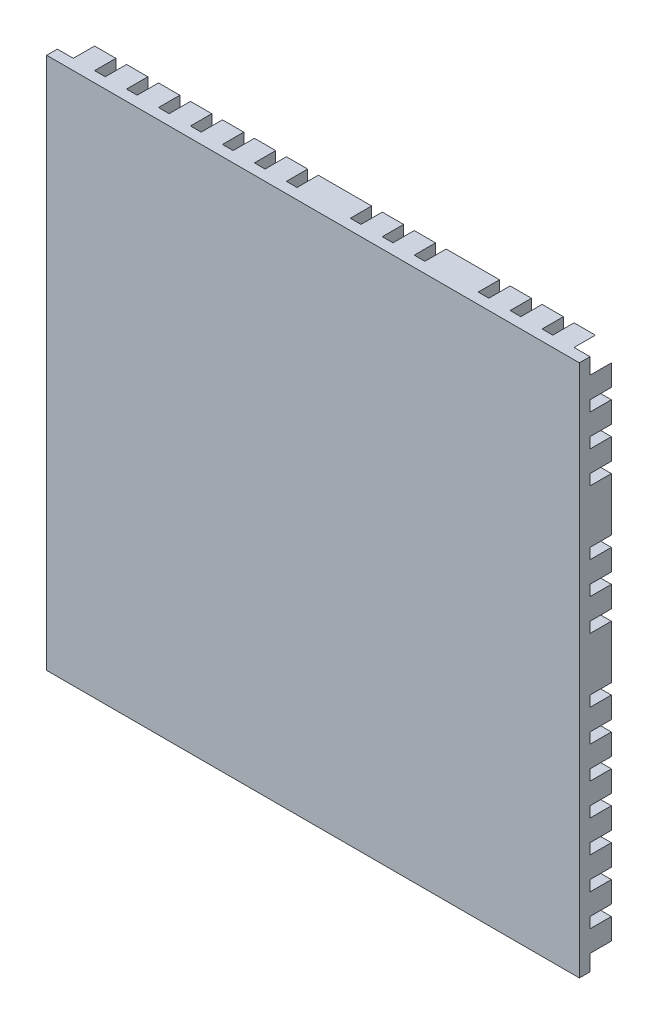
from build123d import *

# Parameters (mm, degrees)
BOSS_EXTRUDE3_DEPTH = 1
SKETCH2_W           = 50
SKETCH2_H           = 50
BOSS_EXTRUDE4_DEPTH = 3
CUT_EXTRUDE1_DEPTH  = 3


with BuildPart() as part:
    # Sketch1 → Boss-Extrude3 (new body)
    with BuildSketch(Plane.XY):
        Polygon((-25, -25), (-23.5, -25), (-21.5, -23), (-21.5, -25), (-20.5, -25), (-20.5, -22), (-18.5, -20), (-18.5, -25), (-17.5, -25), (-17.5, -19), (-15.5, -17), (-15.5, -25), (-14.5, -25), (-14.5, -16), (-12.5, -14), (-12.5, -25.000006046), (-11.5, -25.000006046), (-11.5, -13), (-9.5, -11), (-9.5, -25.000006046), (-8.5, -25.000006046), (-8.5, -10), (-6.5, -8), (-6.5, -25.000006046), (-5.5, -25.000006046), (-5.5, -7), (-3.5, -5), (-3.5, -25.000006046), (-2.5, -25.000006046), (-2.5, -4), (0, -1.5), (2.5, -4), (2.5, -25.000006046), (3.5, -25.000006046), (3.5, -5), (5.5, -7), (5.5, -25.000006046), (6.5, -25.000006046), (6.5, -8), (8.5, -10), (8.5, -25.000006046), (9.5, -25.000006046), (9.5, -11), (11.5, -13), (11.5, -25.000006046), (12.5, -25.000006046), (12.5, -14), (14.5, -16), (14.5, -25), (15.5, -25), (15.5, -17), (17.5, -19), (17.5, -25), (18.5, -25), (18.5, -20), (20.5, -22), (20.5, -25), (21.5, -25), (21.5, -23), (23.5, -25), (25, -25), (25, -23.5), (23, -21.5), (25, -21.5), (25, -20.5), (22, -20.5), (20, -18.5), (25, -18.5), (25, -17.5), (19, -17.5), (17, -15.5), (25, -15.5), (25, -14.5), (16, -14.5), (14, -12.5), (25.000006046, -12.5), (25.000006046, -11.5), (13, -11.5), (11, -9.5), (25.000006046, -9.5), (25.000006046, -8.5), (10, -8.5), (8, -6.5), (25.000006046, -6.5), (25.000006046, -5.5), (7, -5.5), (5, -3.5), (25.000006046, -3.5), (25.000006046, -2.5), (4, -2.5), (1.5, 0), (4, 2.5), (25.000006046, 2.5), (25.000006046, 3.5), (5, 3.5), (7, 5.5), (25.000006046, 5.5), (25.000006046, 6.5), (8, 6.5), (10, 8.5), (25.000006046, 8.5), (25.000006046, 9.5), (11, 9.5), (16, 14.5), (25, 14.5), (25, 15.5), (17, 15.5), (19, 17.5), (25, 17.5), (25, 18.5), (20, 18.5), (22, 20.5), (25, 20.5), (25, 21.5), (23, 21.5), (25, 23.5), (25, 25), (23.5, 25), (21.5, 23), (21.5, 25), (20.5, 25), (20.5, 22), (18.5, 20), (18.5, 25), (17.5, 25), (17.5, 19), (15.5, 17), (15.5, 25), (14.5, 25), (14.5, 16), (9.5, 11), (9.5, 25.000006046), (8.5, 25.000006046), (8.5, 10), (6.5, 8), (6.5, 25.000006046), (5.5, 25.000006046), (5.5, 7), (3.5, 5), (3.5, 25.000006046), (2.5, 25.000006046), (2.5, 4), (0, 1.5), (-2.5, 4), (-2.5, 25.000006046), (-3.5, 25.000006046), (-3.5, 5), (-5.5, 7), (-5.5, 25.000006046), (-6.5, 25.000006046), (-6.5, 8), (-8.5, 10), (-8.5, 25.000006046), (-9.5, 25.000006046), (-9.5, 11), (-11.5, 13), (-11.5, 25.000006046), (-12.5, 25.000006046), (-12.5, 14), (-14.5, 16), (-14.5, 25), (-15.5, 25), (-15.5, 17), (-17.5, 19), (-17.5, 25), (-18.5, 25), (-18.5, 20), (-20.5, 22), (-20.5, 25), (-21.5, 25), (-21.5, 23), (-23.5, 25), (-25, 25), (-25, 23.5), (-23, 21.5), (-25, 21.5), (-25, 20.5), (-22, 20.5), (-20, 18.5), (-25, 18.5), (-25, 17.5), (-19, 17.5), (-17, 15.5), (-25, 15.5), (-25, 14.5), (-16, 14.5), (-14, 12.5), (-25.000006046, 12.5), (-25.000006046, 11.5), (-13, 11.5), (-11, 9.5), (-25.000006046, 9.5), (-25.000006046, 8.5), (-10, 8.5), (-8, 6.5), (-25.000006046, 6.5), (-25.000006046, 5.5), (-7, 5.5), (-5, 3.5), (-25.000006046, 3.5), (-25.000006046, 2.5), (-4, 2.5), (-1.5, 0), (-4, -2.5), (-25.000006046, -2.5), (-25.000006046, -3.5), (-5, -3.5), (-7, -5.5), (-25.000006046, -5.5), (-25.000006046, -6.5), (-8, -6.5), (-10, -8.5), (-25.000006046, -8.5), (-25.000006046, -9.5), (-11, -9.5), (-13, -11.5), (-25.000006046, -11.5), (-25.000006046, -12.5), (-14, -12.5), (-16, -14.5), (-25, -14.5), (-25, -15.5), (-17, -15.5), (-19, -17.5), (-25, -17.5), (-25, -18.5), (-20, -18.5), (-22, -20.5), (-25, -20.5), (-25, -21.5), (-23, -21.5), (-25, -23.5), align=None)
    extrude(amount=BOSS_EXTRUDE3_DEPTH)


with BuildPart() as body_2:
    # Sketch2 → Boss-Extrude4 (new body)
    with BuildSketch(Plane.XY.offset(1)):
        Rectangle(SKETCH2_W, SKETCH2_H)
    extrude(amount=BOSS_EXTRUDE4_DEPTH)


with BuildPart() as cut_extrude1_tool:
    # Sketch3 → Cut-Extrude1 (new body)
    with BuildSketch(Plane(origin=(0, 0, 0), x_dir=(-1, 0, 0), z_dir=(0, 0, -1))):
        Polygon((20.5, -22), (20.5, -25), (21.5, -25), (21.5, -23), (23.5, -25), (25, -25), (25, -23.5), (23, -21.5), (25, -21.5), (25, -20.5), (22, -20.5), (20, -18.5), (25, -18.5), (25, -17.5), (19, -17.5), (17, -15.5), (25, -15.5), (25, -14.5), (16, -14.5), (14, -12.5), (25.000006046, -12.5), (25.000006046, -11.5), (13, -11.5), (11, -9.5), (25.000006046, -9.5), (25.000006046, -8.5), (10, -8.5), (8, -6.5), (25.000006046, -6.5), (25.000006046, -5.5), (7, -5.5), (5, -3.5), (25.000006046, -3.5), (25.000006046, -2.5), (4, -2.5), (1.5, 0), (4, 2.5), (25.000006046, 2.5), (25.000006046, 3.5), (5, 3.5), (7, 5.5), (25.000006046, 5.5), (25.000006046, 6.5), (8, 6.5), (10, 8.5), (25.000006046, 8.5), (25.000006046, 9.5), (11, 9.5), (13, 11.5), (25.000006046, 11.5), (25.000006046, 12.5), (14, 12.5), (16, 14.5), (25, 14.5), (25, 15.5), (17, 15.5), (19, 17.5), (25, 17.5), (25, 18.5), (20, 18.5), (22, 20.5), (25, 20.5), (25, 21.5), (23, 21.5), (25, 23.5), (25, 25), (23.5, 25), (21.5, 23), (21.5, 25), (20.5, 25), (20.5, 22), (18.5, 20), (18.5, 25), (17.5, 25), (17.5, 19), (15.5, 17), (15.5, 25), (14.5, 25), (14.5, 16), (12.5, 14), (12.5, 25.000006046), (11.5, 25.000006046), (11.5, 13), (9.5, 11), (9.5, 25.000006046), (8.5, 25.000006046), (8.5, 10), (6.5, 8), (6.5, 25.000006046), (5.5, 25.000006046), (5.5, 7), (3.5, 5), (3.5, 25.000006046), (2.5, 25.000006046), (2.5, 4), (0, 1.5), (-2.5, 4), (-2.5, 25.000006046), (-3.5, 25.000006046), (-3.5, 5), (-5.5, 7), (-5.5, 25.000006046), (-6.5, 25.000006046), (-6.5, 8), (-8.5, 10), (-8.5, 25.000006046), (-9.5, 25.000006046), (-9.5, 11), (-14.5, 16), (-14.5, 25), (-15.5, 25), (-15.5, 17), (-17.5, 19), (-17.5, 25), (-18.5, 25), (-18.5, 20), (-20.5, 22), (-20.5, 25), (-21.5, 25), (-21.5, 23), (-23.5, 25), (-25, 25), (-25, 23.5), (-23, 21.5), (-25, 21.5), (-25, 20.5), (-22, 20.5), (-20, 18.5), (-25, 18.5), (-25, 17.5), (-19, 17.5), (-17, 15.5), (-25, 15.5), (-25, 14.5), (-16, 14.5), (-11, 9.5), (-25.000006046, 9.5), (-25.000006046, 8.5), (-10, 8.5), (-8, 6.5), (-25.000006046, 6.5), (-25.000006046, 5.5), (-7, 5.5), (-5, 3.5), (-25.000006046, 3.5), (-25.000006046, 2.5), (-4, 2.5), (-1.5, 0), (-4, -2.5), (-25.000006046, -2.5), (-25.000006046, -3.5), (-5, -3.5), (-7, -5.5), (-25.000006046, -5.5), (-25.000006046, -6.5), (-8, -6.5), (-10, -8.5), (-25.000006046, -8.5), (-25.000006046, -9.5), (-11, -9.5), (-13, -11.5), (-25.000006046, -11.5), (-25.000006046, -12.5), (-14, -12.5), (-16, -14.5), (-25, -14.5), (-25, -15.5), (-17, -15.5), (-19, -17.5), (-25, -17.5), (-25, -18.5), (-20, -18.5), (-22, -20.5), (-25, -20.5), (-25, -21.5), (-23, -21.5), (-25, -23.5), (-25, -25), (-23.5, -25), (-21.5, -23), (-21.5, -25), (-20.5, -25), (-20.5, -22), (-18.5, -20), (-18.5, -25), (-17.5, -25), (-17.5, -19), (-15.5, -17), (-15.5, -25), (-14.5, -25), (-14.5, -16), (-12.5, -14), (-12.5, -25.000006046), (-11.5, -25.000006046), (-11.5, -13), (-9.5, -11), (-9.5, -25.000006046), (-8.5, -25.000006046), (-8.5, -10), (-6.5, -8), (-6.5, -25.000006046), (-5.5, -25.000006046), (-5.5, -7), (-3.5, -5), (-3.5, -25.000006046), (-2.5, -25.000006046), (-2.5, -4), (0, -1.5), (2.5, -4), (2.5, -25.000006046), (3.5, -25.000006046), (3.5, -5), (5.5, -7), (5.5, -25.000006046), (6.5, -25.000006046), (6.5, -8), (8.5, -10), (8.5, -25.000006046), (9.5, -25.000006046), (9.5, -11), (11.5, -13), (11.5, -25.000006046), (12.5, -25.000006046), (12.5, -14), (14.5, -16), (14.5, -25), (15.5, -25), (15.5, -17), (17.5, -19), (17.5, -25), (18.5, -25), (18.5, -20), align=None)
    extrude(amount=-CUT_EXTRUDE1_DEPTH)


with BuildPart() as part_1:
    add(part.part)

    # Cut-Extrude1: cut by cut_extrude1_tool
    add(cut_extrude1_tool.part, mode=Mode.SUBTRACT)


with BuildPart() as body_2_1:
    add(body_2.part)

    # Cut-Extrude1: cut by cut_extrude1_tool
    add(cut_extrude1_tool.part, mode=Mode.SUBTRACT)


solid = body_2_1.part
